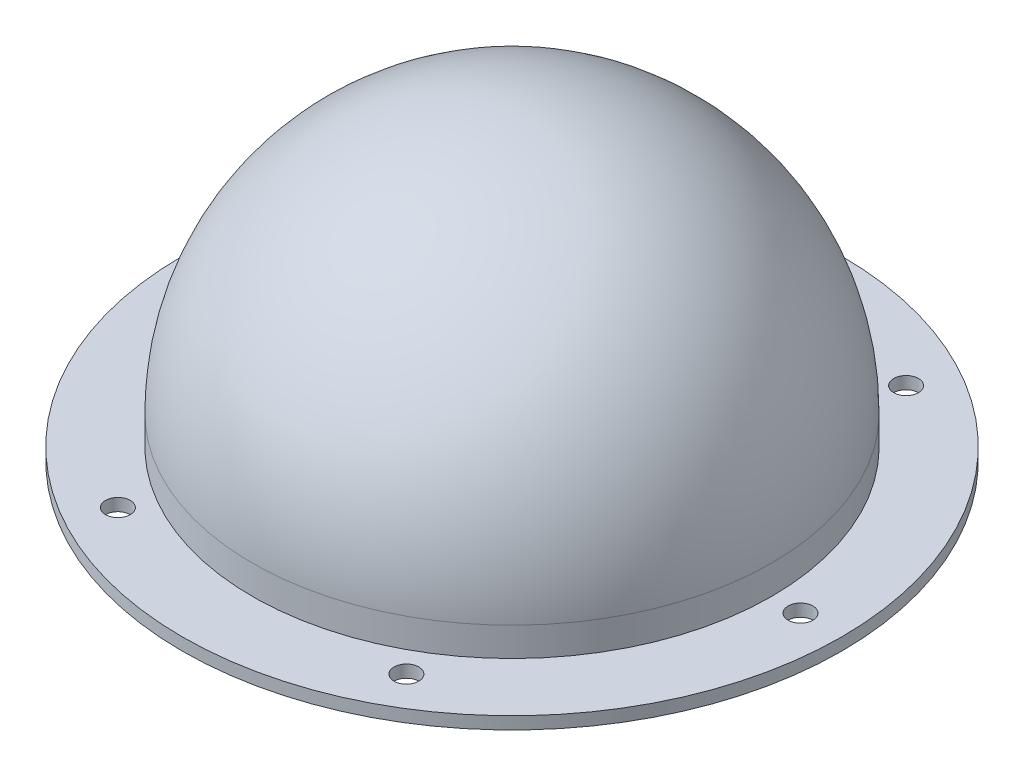
SolidWorks part; units mm, degrees
ref_plane "Front Plane" through (0, 0, 0) normal (0, 0, 1) x (1, 0, 0)
ref_plane "Top Plane" through (0, 0, 0) normal (0, 1, 0) x (1, 0, 0)
ref_plane "Right Plane" through (0, 0, 0) normal (1, 0, 0) x (0, 0, -1)
sketch "Sketch1" plane through (0, 0, 0) normal (0, 0, 1) x (1, 0, 0)
  line L0 (0, 19.3816) -> (0, 39.5691) construction
  line L1 (-40, 0) -> (-30, 0)
  line L2 (-30, 0) -> (-30, 5)
  line L3 (-31.5, 1.5) -> (-31.5, 5)
  line L4 (-40, 1.5) -> (-31.5, 1.5)
  line L5 (-40, 1.5) -> (-40, 0)
  line L6 (0, 35) -> (0, 36.5)
  arc A0 (0, 35) -> (-30, 5) centre (0, 5) ccw
  arc A1 (0, 36.5) -> (-31.5, 5) centre (0, 5) ccw
  dimension "D2" = 60
  dimension "D1" = 10
  dimension "D3" = 30
  dimension "D4" = 5
  dimension "D5" = 1.5
revolve "Revolve1" add sketch "Sketch1" angle 360 about L6
sketch "Sketch2" plane through (0, 1.5, 0) normal (0, 1, 0) x (1, 0, 0)
  circle A0 centre (0, 0) radius 35 construction
  circle A1 centre (-35, 0) radius 1.5
  circle A2 centre (-17.5, 30.3109) radius 1.5
  circle A3 centre (17.5, 30.3109) radius 1.5
  circle A4 centre (35, 0) radius 1.5
  circle A5 centre (17.5, -30.3109) radius 1.5
  circle A6 centre (-17.5, -30.3109) radius 1.5
  point P17 (0, 0)
  dimension "D1" = 70
  dimension "D2" = 3
  dimension "D3" = 6
extrude "Cut-Extrude1" cut sketch "Sketch2" against normal through all
